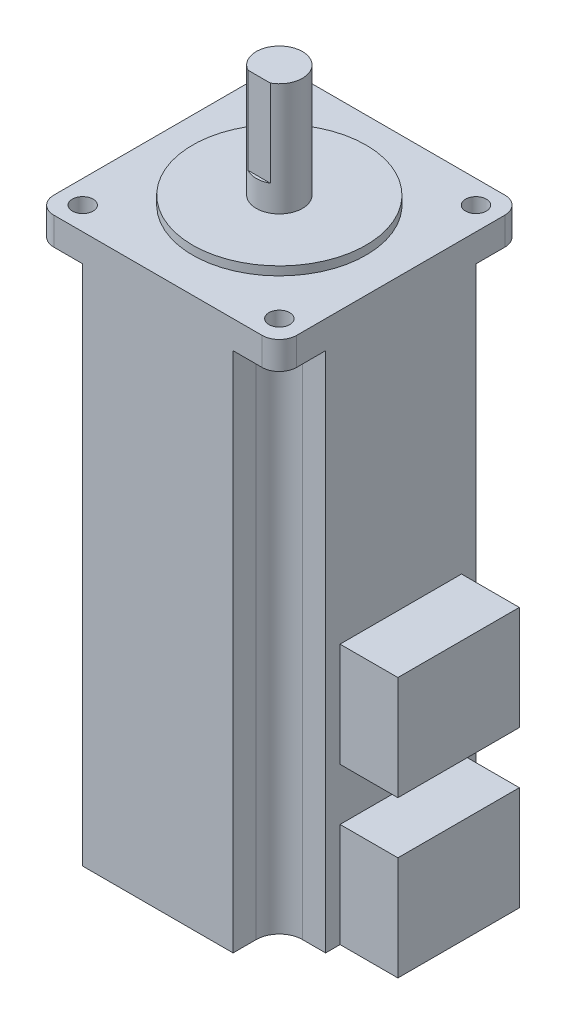
SolidWorks part; units mm, degrees
ref_plane "Front Plane" through (0, 0, 0) normal (0, 0, 1) x (1, 0, 0)
ref_plane "Top Plane" through (0, 0, 0) normal (0, 1, 0) x (1, 0, 0)
ref_plane "Right Plane" through (0, 0, 0) normal (1, 0, 0) x (0, 0, -1)
sketch "Sketch1" plane through (0, 0, 0) normal (0, 1, 0) x (1, 0, 0)
  line L1 (-21, -21) -> (21, -21)
  line L2 (-21, -21) -> (-21, 21)
  line L3 (-21, 21) -> (21, 21)
  line L4 (21, -21) -> (21, 21)
  line L5 (-21, -21) -> (21, 21) construction
  line L6 (-21, 21) -> (21, -21) construction
  point P0 (0, 0)
  dimension "D1" = 42
  dimension "D2" = 42
extrude "Boss-Extrude1" add sketch "Sketch1" along normal blind 95
sketch "Sketch2" plane through (0, 0, 0) normal (0, -1, 0) x (1, 0, 0)
  line L1 (-21, 21) -> (-13, 21)
  line L2 (-21, 21) -> (-21, 13)
  line L3 (-21, 13) -> (-13, 13)
  line L4 (-13, 21) -> (-13, 13)
  line L5 (21, 21) -> (13, 21)
  line L6 (21, 21) -> (21, 13)
  line L7 (21, 13) -> (13, 13)
  line L8 (13, 21) -> (13, 13)
  line L9 (-21, -21) -> (-13, -21)
  line L10 (-21, -21) -> (-21, -13)
  line L11 (-21, -13) -> (-13, -13)
  line L12 (-13, -21) -> (-13, -13)
  line L13 (21, -21) -> (13, -21)
  line L14 (21, -21) -> (21, -13)
  line L15 (21, -13) -> (13, -13)
  line L16 (13, -21) -> (13, -13)
  dimension "D1" = 8
extrude "Cut-Extrude1" cut sketch "Sketch2" against normal offset from surface (90.2 mm away) 4.8 up to face at (0, 95, 0)
sketch "Sketch3" plane through (0, 95, 0) normal (0, 1, 0) x (1, 0, 0)
  line L1 (17, -17) -> (-17, -17) construction
  line L2 (17, -17) -> (17, 17) construction
  line L3 (17, 17) -> (-17, 17) construction
  line L4 (-17, -17) -> (-17, 17) construction
  line L5 (17, -17) -> (-17, 17) construction
  line L6 (17, 17) -> (-17, -17) construction
  circle A0 centre (-17, 17) radius 1.8
  circle A1 centre (17, 17) radius 1.8
  circle A2 centre (-17, -17) radius 1.8
  circle A3 centre (17, -17) radius 1.8
  point P8 (0, 0)
  dimension "D2" = 3.6
  dimension "D1" = 34
extrude "Cut-Extrude2" cut sketch "Sketch3" against normal blind 4.8
fillet "Fillet1" radius 4 4 edges at (13, 45.1, 13) (-13, 45.1, 13) (-13, 45.1, -13) (13, 45.1, -13)
sketch "Sketch4" plane through (0, 95, 0) normal (0, 1, 0) x (1, 0, 0)
  circle A0 centre (0, 0) radius 15
  dimension "D1" = 30
extrude "Boss-Extrude2" add sketch "Sketch4" along normal blind 1.5
sketch "Sketch5" plane through (0, 95, 0) normal (0, 1, 0) x (1, 0, 0)
  circle A0 centre (0, 0) radius 4
  dimension "D1" = 8
extrude "Boss-Extrude3" add sketch "Sketch5" along normal blind 21
fillet "Fillet2" radius 3 4 edges at (-21, 92.6, -21) (-21, 92.6, 21) (21, 92.6, 21) (21, 92.6, -21)
sketch "Sketch7" plane through (0, 0, 0) normal (0, -1, 0) x (1, 0, 0)
  circle A0 centre (0, 0) radius 21
  dimension "D1" = 42
extrude "Boss-Extrude4" [suppressed] add sketch "Sketch7" along normal blind 28
sketch "Sketch8" plane through (21, 0, 0) normal (1, 0, 0) x (0, 0, -1)
  line L0 (-13, 0) -> (13, 0) construction
  line L1 (10.5, 0) -> (-10.5, 0)
  line L2 (10.5, 0) -> (10.5, 18)
  line L3 (10.5, 18) -> (-10.5, 18)
  line L4 (-10.5, 0) -> (-10.5, 18)
  line L5 (0, 0) -> (0, -22.6807) construction
  line L7 (-10.5, 45) -> (10.5, 45)
  line L8 (-10.5, 45) -> (-10.5, 27)
  line L9 (-10.5, 27) -> (10.5, 27)
  line L10 (10.5, 45) -> (10.5, 27)
  dimension "D1" = 18
  dimension "D2" = 21
  dimension "D3" = 45
  dimension "D4" = 18
extrude "Boss-Extrude5" add sketch "Sketch8" along normal blind 10
sketch "Sketch9" plane through (0, 116, 0) normal (0, 1, 0) x (1, 0, 0)
  line L1 (5.451, -7.5113) -> (-8.2652, -7.5113)
  line L2 (5.451, -7.5113) -> (5.451, -3.5)
  line L3 (5.451, -3.5) -> (-8.2652, -3.5)
  line L4 (-8.2652, -7.5113) -> (-8.2652, -3.5)
  circle A0 centre (0, 0) radius 4 construction
  dimension "D1" = 3.5
extrude "Cut-Extrude3" cut sketch "Sketch9" against normal blind 15
